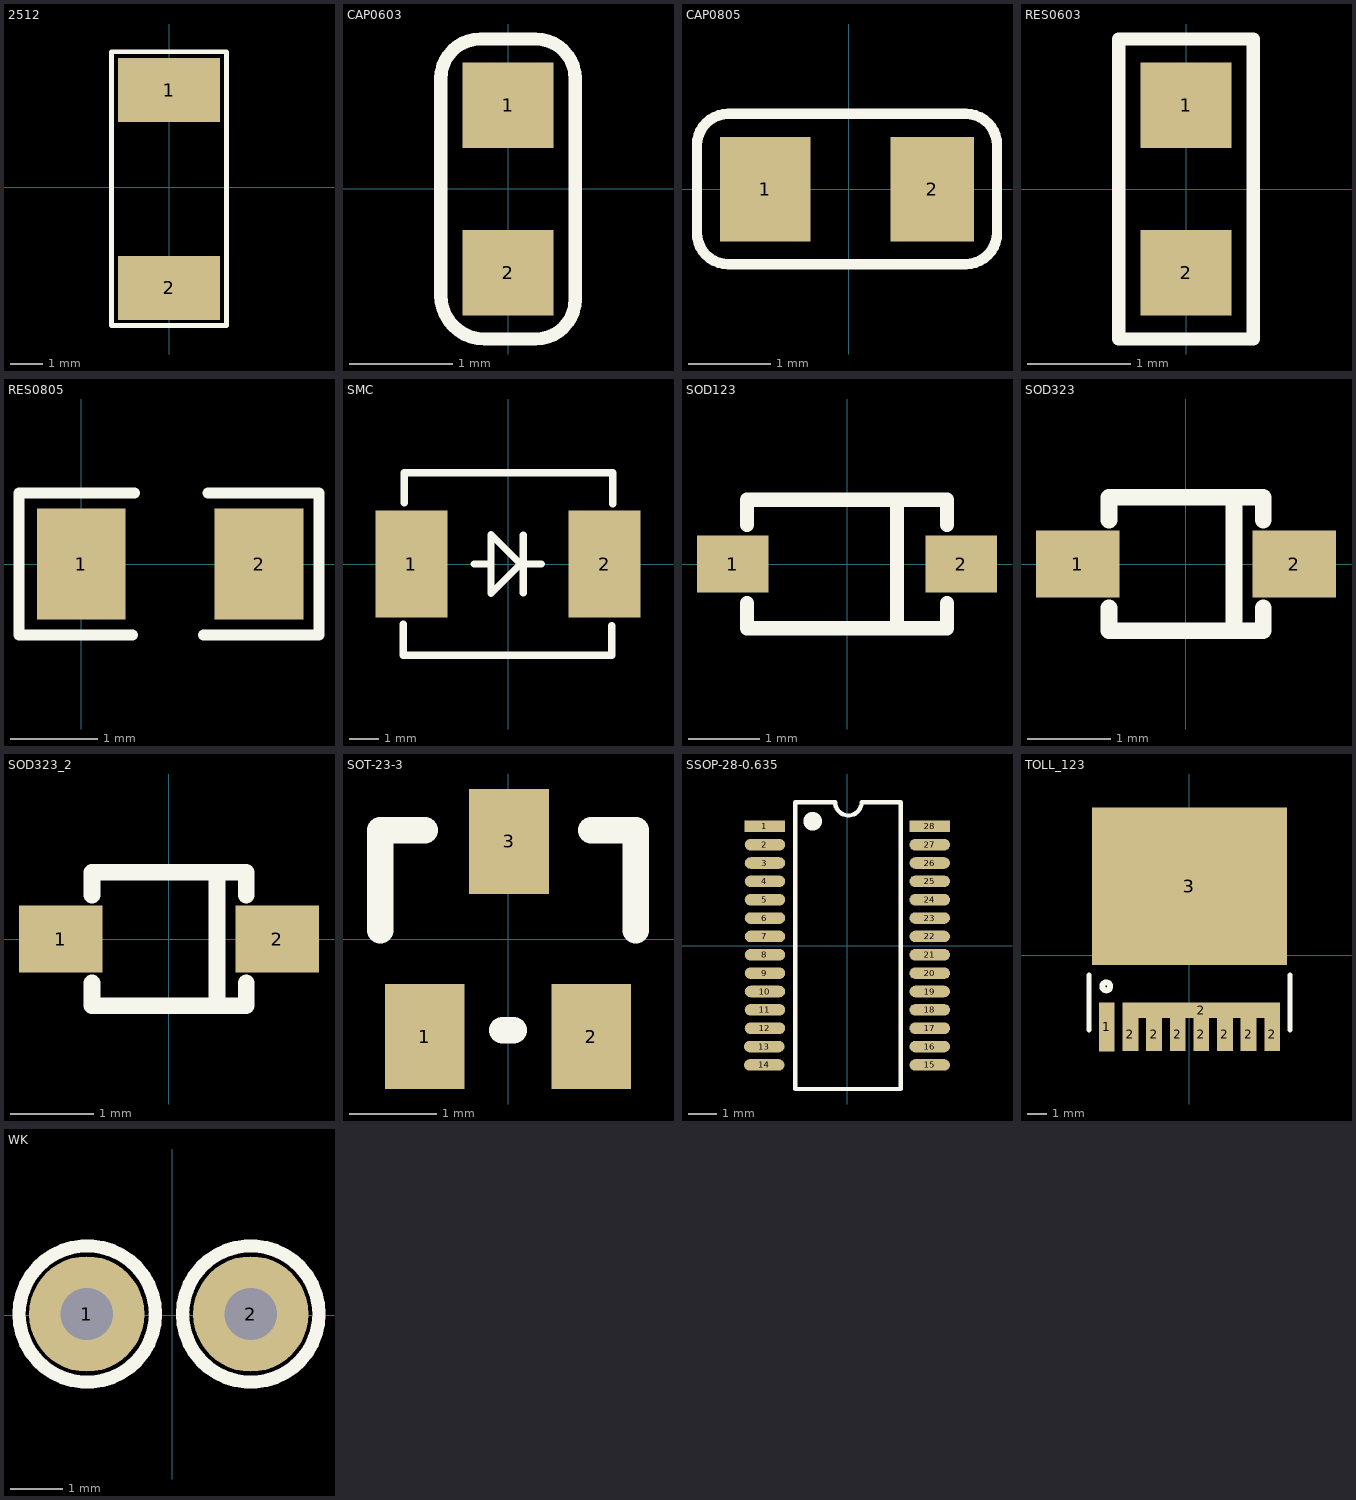
[diagram p0: the footprints below, top view; thin cyan lines are the x and y axes]
# Altium footprint library MISC84391-2.PcbLib: 13 footprints
Each footprint in its own frame and in the unit in brackets; x right, y up, seen from the top. Pads: shape width x height; smd on the part's side, far side on the other; paste and mask are expansions set on the pad; w line width, h text height; cw(c..) or ccw(c..) is an arc to the next point about the centre after c.

## 2512 [mm]
height 1.2
pads (2):
  rect 3.2x2 smd: 1(0,3.05) 2(0,-3.15)
Top Overlay:
  lines w0.15: -1.802,-4.325 -1.802,4.25 1.801,4.25 1.801,-4.325 -1.802,-4.325

## CAP0603 [mm] "CAP0402"
height 3.35
pads (2):
  rect 0.88x0.83 smd mask+0: 1(0,0.81) 2(0,-0.81)
Top Overlay:
  lines w0.127: -0.65,-1.027 ccw(c-0.227,-1.027) -0.227,-1.45 0.267,-1.45 ccw(c0.267,-1.067) 0.65,-1.067 0.65,1.067 ccw(c0.267,1.067) 0.267,1.45 -0.267,1.45 ccw(c-0.267,1.067) -0.65,1.067 -0.65,-1.027
3D body "0603_C.step": height 0.88, standoff 0, extent -0.412,-0.791 0.398,0.809

## CAP0805 [mil]
height 100
pads (2):
  rect 43.31x50 smd: 1(-40,0)
  rect 40x50 smd: 2(40,0)
Top Overlay:
  lines w5: 56,-35.96 -57.66,-35.96 cw(c-57.66,-21) -72.62,-21 -72.62,21 cw(c-57.66,21) -57.66,35.96 56,35.96 ; 56,-35.92 ccw(c56,-20.96) 70.96,-20.96 70.96,21.04 ccw(c56,21.04) 56,36
3D body "0805 SMD Capacitor.STEP": height 34.72, standoff 3.94, extent -39.36,-24.6 39.38,24.61

## RES0603 [mm] "CAP0402"
height 3.35
pads (2):
  rect 0.88x0.83 smd mask+0: 1(0,0.81) 2(0,-0.81)
Top Overlay:
  lines w0.127: 0.64,-1.45 -0.65,-1.45 -0.65,-0.4 -0.65,1.45 0.65,1.45 0.65,-0.44 ; 0.65,-1.45 0.65,-0.4
3D body "0603res.stp": height 0.3, standoff 0, extent -0.4,-0.83 0.4,0.77

## RES0805 [mil]
height 100
pads (2):
  rect 40x50 smd: 1(0,0) 2(80,0)
Top Overlay:
  lines w5: 23,-32 -28,-32 -28,32 24,32 ; 55,-32 107,-32 107,32 57,32
3D body "RES0805.STEP": height 3.94, standoff -12.2, extent 0.63,-25 79.37,24.21

## SMC [mm]
height 1.35
pads (2):
  rect 2.44x3.62 smd: 1(-3.275,0) 2(3.275,0)
Top Overlay:
  lines w0.25: -0.575,-1 0.425,0 -0.575,1 -0.575,-1
  lines w0.254: -3.55,-3.1 3.525,-3.1 3.525,-2.1 ; -3.55,-3.075 -3.55,-2.05 ; -3.525,2.075 -3.525,3.1 3.55,3.1 3.55,2.05 ; -1.15,0 -0.6,0 ; 0.5,0 1.125,0 ; 0.525,-0.975 0.525,0.025 ; 0.525,0 0.525,0.975

## SOD123 [mm]
height 2.45
pads (2):
  rect 1x0.8 smd: 1(-1.6,0) 2(1.6,0)
Top Overlay:
  lines w0.2: -1.4,-0.55 -1.4,-0.9 1.4,-0.9 1.4,-0.55 ; -1.4,0.55 -1.4,0.9 1.4,0.9 1.4,0.55 ; 0.7,-0.8 0.7,-0.5 0.7,0.8

## SOD323 [mm]
height 2.45
pads (2):
  rect 1x0.8 smd: 1(-1.3,0) 2(1.3,0)
Top Overlay:
  lines w0.2: -0.924,-0.525 -0.924,-0.8 0.926,-0.8 0.926,-0.525 ; -0.924,0.525 -0.924,0.8 0.926,0.8 0.926,0.525 ; 0.576,-0.8 0.576,-0.5 0.576,0.8

## SOD323_2 [mm]
pads (2):
  rect 1x0.8 smd: 1(-1.3,0) 2(1.3,0)
Top Overlay:
  lines w0.2: -0.924,-0.525 -0.924,-0.8 0.926,-0.8 0.926,-0.525 ; -0.924,0.525 -0.924,0.8 0.926,0.8 0.926,0.525 ; 0.576,-0.8 0.576,-0.5 0.576,0.8

## SOT-23-3 [mil]
height 55.12
pads (3):
  rect 36x47.24 smd: 1(-37.5,-43.94) 2(37.5,-43.94) 3(0.5,43.94)
Top Overlay:
  lines w12: -57.5,3.94 -57.5,48.94 -37.5,48.94 ; -2.5,-41.06 2.5,-41.06 ; 37.5,48.94 57.5,48.94 57.5,3.94

## SSOP-28-0.635 [mm]
height 1.4
pads (28):
  rect 1.4x0.4 smd: 1(-2.838,4.127) 28(2.862,4.127)
  oval 1.4x0.4 smd: 2(-2.838,3.492) 3(-2.838,2.857) 4(-2.838,2.222) 5(-2.838,1.587) 6(-2.838,0.953) 7(-2.838,0.318) 8(-2.838,-0.318) 9(-2.838,-0.953) 10(-2.838,-1.587) 11(-2.838,-2.222) 12(-2.838,-2.857) 13(-2.862,-3.492) 14(-2.862,-4.127) 15(2.862,-4.127) 16(2.862,-3.492) 17(2.862,-2.857) 18(2.862,-2.222) 19(2.862,-1.587) 20(2.862,-0.953) 21(2.862,-0.318) 22(2.862,0.318) 23(2.862,0.953) 24(2.862,1.587) 25(2.862,2.222) 26(2.862,2.857) 27(2.862,3.492)
Top Overlay:
  circle w0.5: c-1.188,4.303 r0.071
  lines w0.15: -1.787,4.96 -1.787,-4.96 1.863,-4.96 1.863,4.96 0.506,4.96 cw(c0.048,4.96) -0.41,4.96 -1.78,4.96

## TOLL_123 [mm] "SMD MOSFET"
height 3.35
pads (10):
  rect 0.8x2.5 smd: 1(-4.2,-3.638)
  rect 0.8x1.7 smd: 2(-3,-4) 2(-1.8,-4) 2(-0.6,-4) 2(0.6,-4) 2(1.8,-4) 2(3,-4) 2(4.2,-4)
  rect 8x0.8 smd: 2(0.6,-2.788)
  rect 9.9x8 smd: 3(0,3.5)
Top Overlay:
  circle w0.3: c-4.225,-1.575 r0.2
  lines w0.254: -5.1,-3.8 -5.1,-1 ; 5.1,-3.8 5.1,-1
Top Paste:
  region: -3.4,-3.03 -3.4,-2.39 4.6,-2.39 4.6,-3.08
  region: -4.95,7.5 4.95,7.5 4.95,-0.5 -4.95,-0.5
  region: -4.6,-4.85 -4.6,-3.15 -3.8,-3.15 -3.8,-4.85
  region: 3.8,-4.85 3.8,-3.25 4.6,-3.25 4.6,-4.85
  region: 2.6,-4.85 2.6,-3.25 3.4,-3.25 3.4,-4.85
  region: 1.4,-4.85 1.4,-3.25 2.2,-3.25 2.2,-4.85
  region: 0.2,-4.85 0.2,-3.25 1,-3.25 1,-4.85
  region: -1,-4.85 -1,-3.25 -0.2,-3.25 -0.2,-4.85
  region: -2.2,-4.85 -2.2,-3.25 -1.4,-3.25 -1.4,-4.85
  region: -3.4,-4.85 -3.4,-3.25 -2.6,-3.25 -2.6,-4.85

## WK [mm]
height 2.45
pads (2):
  round 2.2 hole 1: 1(-1.625,0.025) 2(1.5,0.025)
Top Overlay:
  circle w0.254: c-1.618,0.025 r1.3
  circle w0.254: c1.5,0.025 r1.3